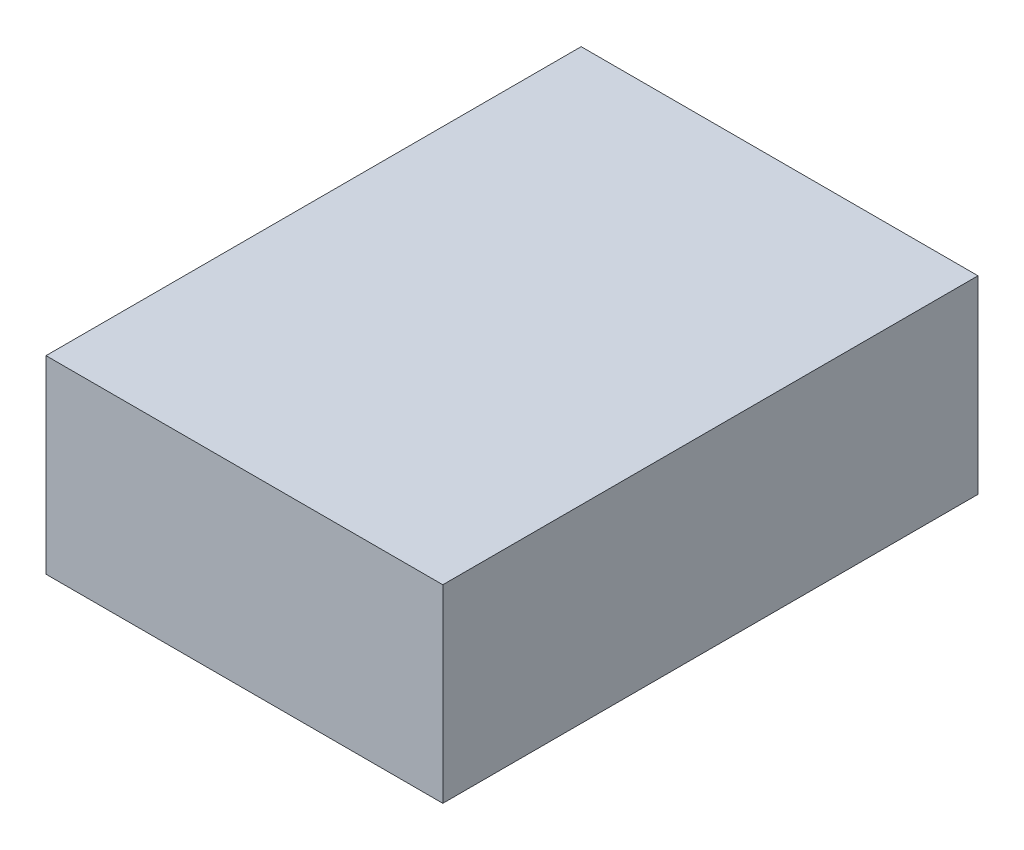
from build123d import *

# Parameters (mm, degrees)
SKETCH_1_W      = 735
SKETCH_1_H      = 260
EXTRUDE_1_DEPTH = 272.5


with BuildPart() as part:
    # 草图1 → 凸台-拉伸1 (new, symmetric)
    with BuildSketch(Plane(origin=(0, 0, 0), x_dir=(0, 0, -1), z_dir=(1, 0, 0))):
        Rectangle(SKETCH_1_W, SKETCH_1_H)
    extrude(amount=EXTRUDE_1_DEPTH, both=True)


solid = part.part
